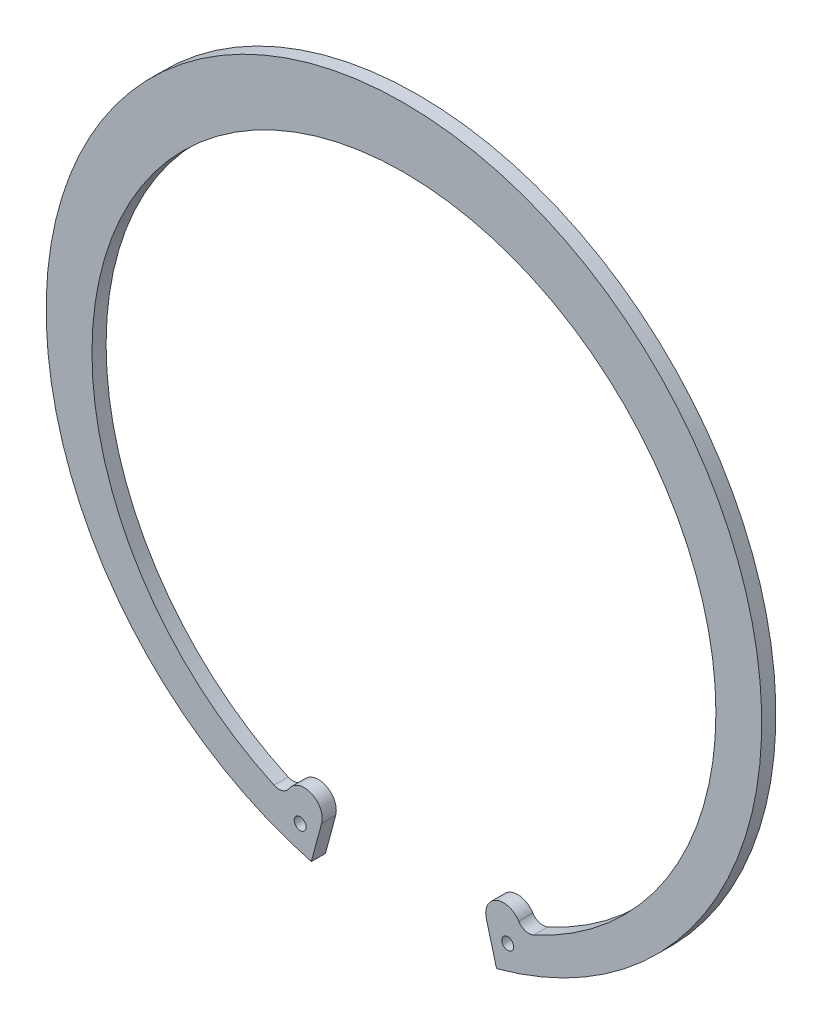
SolidWorks part; units mm, degrees
material "65Mn"
ref_plane "Front Plane" through (0, 0, 0) normal (0, 0, 1) x (1, 0, 0)
ref_plane "Top Plane" through (0, 0, 0) normal (0, 1, 0) x (1, 0, 0)
ref_plane "Right Plane" through (0, 0, 0) normal (1, 0, 0) x (0, 0, -1)
sketch "Dimension sketch" plane through (0, 0, 0) normal (0, 0, 1) x (1, 0, 0)
  line L0 (-120.25, 0) -> (120.25, 0) construction
  line L1 (0, 0) -> (-104.1396, -60.125) construction
  circle A0 centre (0, 0) radius 120.25
  point P5 (-69.45, 0)
  point P6 (94.5, 0)
  point P7 (6, 0)
  point P8 (97.5, 0)
  point P10 (-10.1, 0)
  point P11 (-3.3, 0)
  point P12 (-14.1, 0)
  point P13 (-72.45, 0)
  point P14 (-78.1588, -45.125)
  dimension "DD" = 240.5
  dimension "d" = 189.7
  dimension "RR" = 97.5
  dimension "R1" = 6
  dimension "R2" = 3
  dimension "aa" = 30
  dimension "a" = 14.1
  dimension "d1" = 4
  dimension "c" = 3.3
  dimension "s" = 3
sketch "Sketch1" plane through (0, 0, 0) normal (0, 0, 1) x (1, 0, 0)
  line L0 (0, 120.25) -> (0, -116.1526) construction
  line L1 (-27.6889, -103.3366) -> (-31.123, -116.1526)
  line L2 (-36.258, -112.1345) -> (-33.4845, -101.7836) construction
  line L3 (0, 0) -> (-31.123, -116.1526) construction
  line L4 (27.6889, -103.3366) -> (31.123, -116.1526)
  arc A0 (31.123, -116.1526) -> (-31.123, -116.1526) centre (0, 0) ccw
  arc A1 (43.6394, -100.1369) -> (-43.6394, -100.1369) centre (0, -4.8) ccw
  circle A2 centre (-34.8713, -106.9591) radius 2
  arc A3 (-27.6889, -103.3366) -> (-38.5785, -98.6134) centre (-33.4845, -101.7836) ccw
  arc A4 (-38.5785, -98.6134) -> (-43.6394, -100.1369) centre (-41.9746, -96.4998) cw
  circle A5 centre (34.8713, -106.9591) radius 2
  arc A6 (27.6889, -103.3366) -> (38.5785, -98.6134) centre (33.4845, -101.7836) cw
  arc A7 (38.5785, -98.6134) -> (43.6394, -100.1369) centre (41.9746, -96.4998) ccw
  dimension "D1" = 240.5
  dimension "D2" = 209.7
  dimension "D5" = 4
  dimension "D7" = 6
  dimension "D8" = 4
  dimension "D9" = 19.1
  dimension "D3" = 4.8
  dimension "D4" = 15
  dimension "D6" = 112.5
extrude "Base-Extrude" add sketch "Sketch1" along normal mid plane 4.75
